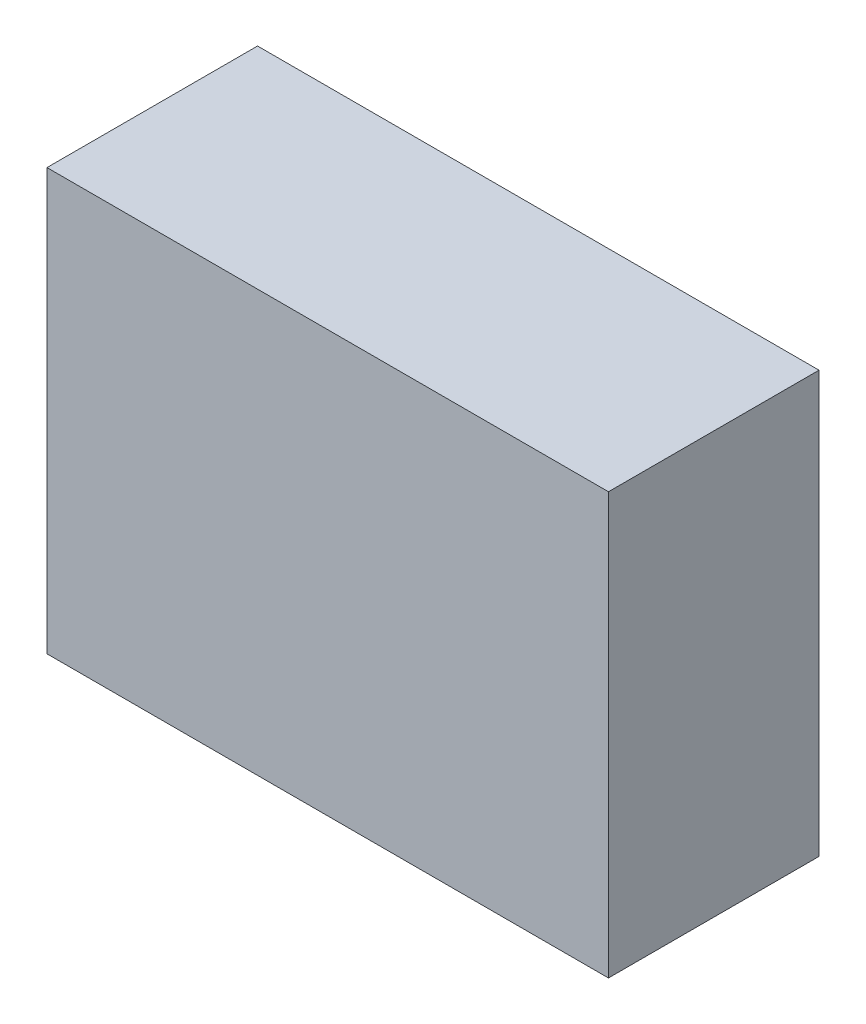
SolidWorks part; units mm, degrees
ref_plane "前视基准面" through (0, 0, 0) normal (0, 0, 1) x (1, 0, 0)
ref_plane "上视基准面" through (0, 0, 0) normal (0, 1, 0) x (1, 0, 0)
ref_plane "右视基准面" through (0, 0, 0) normal (1, 0, 0) x (0, 0, -1)
other "Configuration Table"
sketch "草图1" plane through (0, 0, 0) normal (0, 0, 1) x (1, 0, 0)
  line L0 (-16, -12) -> (16, -12)
  line L1 (16, -12) -> (16, 12)
  line L2 (16, 12) -> (-16, 12)
  line L3 (-16, 12) -> (-16, -12)
  point P0 (0, 0)
  dimension "D1" = 16
  dimension "D2" = 32
  dimension "D3" = 12
  dimension "D4" = 24
extrude "凸台-拉伸1" add sketch "草图1" against normal mid plane 12
